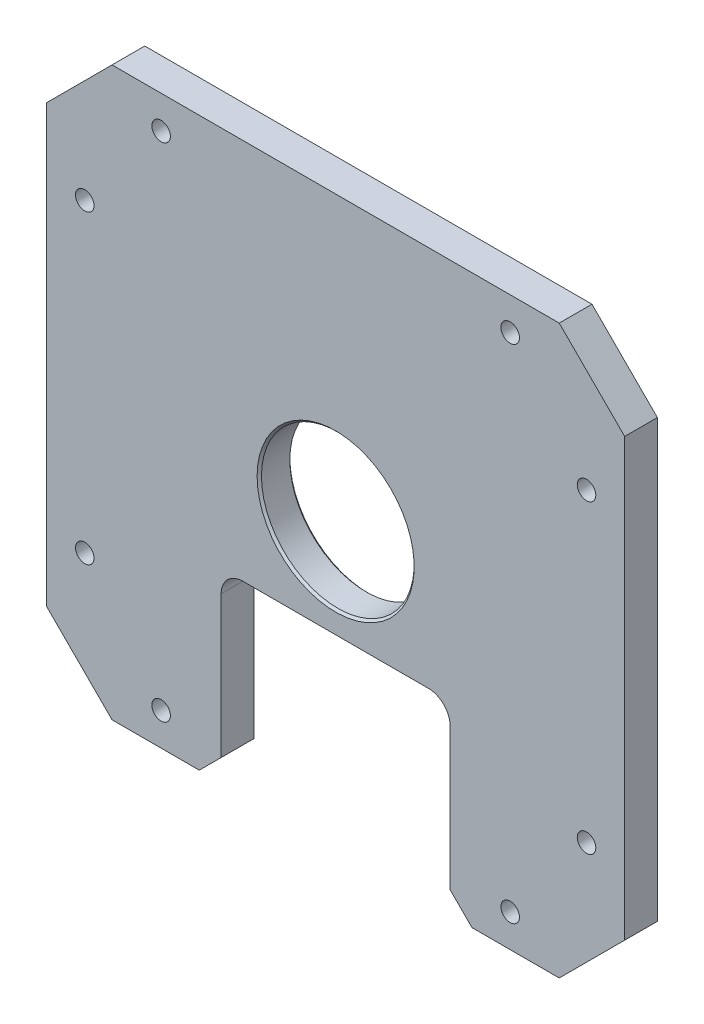
SolidWorks part; units mm, degrees
material "Q235A"
ref_plane "前视基准面" through (0, 0, 0) normal (0, 0, 1) x (1, 0, 0)
ref_plane "上视基准面" through (0, 0, 0) normal (0, 1, 0) x (1, 0, 0)
ref_plane "右视基准面" through (0, 0, 0) normal (1, 0, 0) x (0, 0, -1)
sketch "草图1" plane through (0, 0, 0) normal (0, 0, 1) x (1, 0, 0)
  line L1 (-132.5, -130) -> (132.5, -130)
  line L2 (-132.5, -130) -> (-132.5, 130)
  line L3 (-132.5, 130) -> (132.5, 130)
  line L4 (132.5, -130) -> (132.5, 130)
  line L5 (-132.5, -130) -> (132.5, 130) construction
  line L6 (-132.5, 130) -> (132.5, -130) construction
  point P0 (0, 0)
  dimension "D1" = 265
  dimension "D2" = 260
extrude "凸台-拉伸1" add sketch "草图1" along normal blind 15
hole_wizard "M10 螺纹孔1" positions "草图2" profile "草图3" tap size "M10" standard "ISO" end condition up to next
sketch "草图2" plane through (0, 0, 0) normal (0, 0, -1) x (-1, 0, 0)
  point P0 (-80, 115)
  point P3 (-115, 70)
  point P6 (-115, -70)
  point P9 (-80, -115)
  point P12 (80, -115)
  point P15 (115, -70)
  point P18 (115, 70)
  point P21 (80, 115)
sketch "草图3" plane through (80, 115, 0) normal (1, 0, 0) x (0, 1, 0)
  line L0 (0, 0) -> (0, 15)
  line L1 (0, 15) -> (4.25, 15)
  line L2 (4.25, 15) -> (4.25, 0)
  line L5 (4.25, 0) -> (0, 0)
  line L11 (0, -6.35) -> (0, 107.95) construction
  dimension "通孔螺纹孔钻头直径" = 8.5
  dimension "通孔螺纹孔钻头深度" = 15
cosmetic thread "孔螺蚊线2" parameters "D2"=10
cosmetic thread "孔螺蚊线3" parameters "D2"=10
cosmetic thread "孔螺蚊线4" parameters "D2"=10
cosmetic thread "孔螺蚊线5" parameters "D2"=10
cosmetic thread "孔螺蚊线6" parameters "D2"=10
cosmetic thread "孔螺蚊线7" parameters "D2"=10
cosmetic thread "孔螺蚊线8" parameters "D2"=10
cosmetic thread "孔螺蚊线9" parameters "D2"=10
sketch "草图4" plane through (0, 0, 0) normal (0, 0, -1) x (-1, 0, 0)
  line L0 (0, 0) -> (0, -130) construction
  line L1 (132.5, -130) -> (-132.5, -130) construction
  line L3 (-52.5, -130) -> (52.5, -130)
  line L4 (-52.5, -130) -> (-52.5, -45)
  line L5 (-52.5, -45) -> (52.5, -45)
  line L6 (52.5, -130) -> (52.5, -45)
  dimension "D1" = 105
  dimension "D2" = 85
extrude "切除-拉伸1" cut sketch "草图4" against normal through all
fillet "圆角1" radius 10 2 edges at (-52.5, -45, 7.5) (52.5, -45, 7.5)
sketch "草图5" plane through (0, 0, 0) normal (0, 0, -1) x (-1, 0, 0)
  line L0 (-132.5, 130) -> (132.5, 130) construction
  circle A0 centre (0, 0) radius 35
  dimension "D1" = 130
  dimension "D2" = 70
extrude "切除-拉伸2" cut sketch "草图5" against normal through all
chamfer "倒角2" distance 1 angle 45 2 edges at (-35, 0, 0) (-35, 0, 15)
chamfer "倒角1" distance 30 angle 45 4 edges at (132.5, -130, 7.5) (-132.5, -130, 7.5) (-132.5, 130, 7.5) (132.5, 130, 7.5)
chamfer "倒角3" distance 10 angle 45 2 edges at (-52.5, -130, 7.5) (52.5, -130, 7.5)
